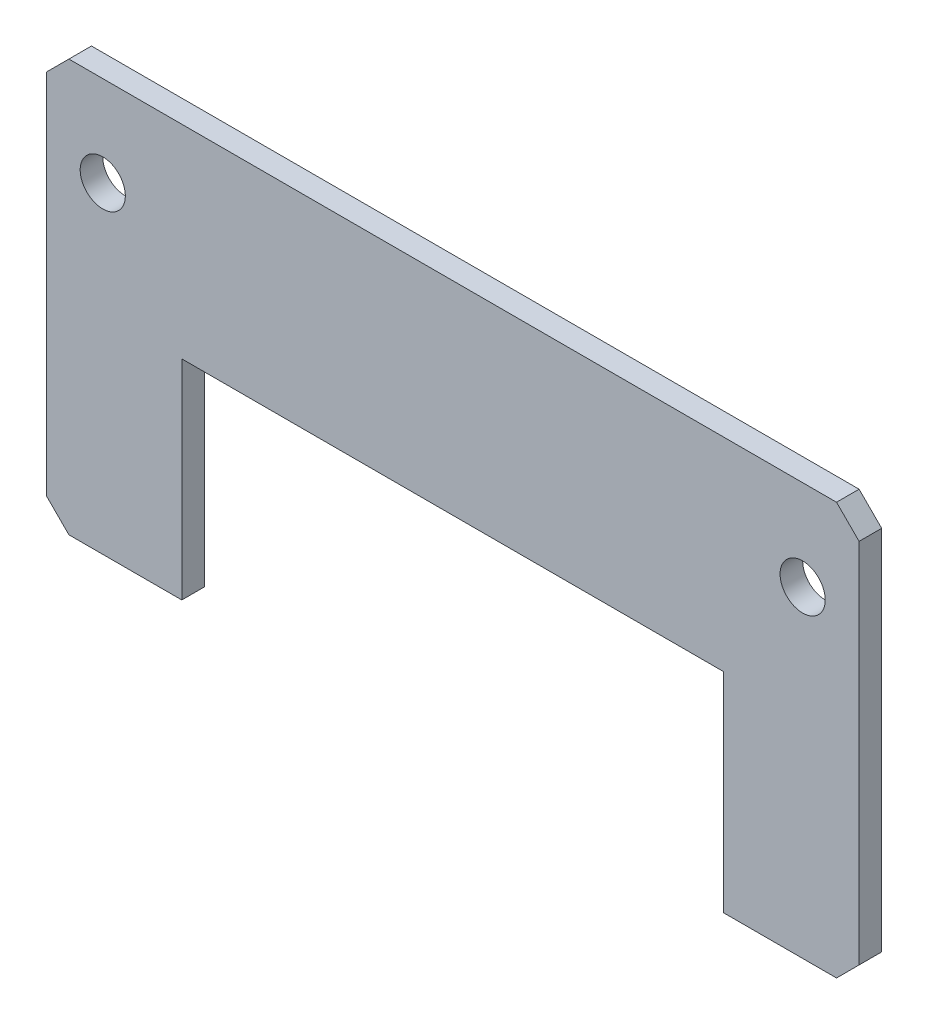
SolidWorks part; units mm, degrees
ref_plane "Front Plane" through (0, 0, 0) normal (0, 0, 1) x (1, 0, 0)
ref_plane "Top Plane" through (0, 0, 0) normal (0, 1, 0) x (1, 0, 0)
ref_plane "Right Plane" through (0, 0, 0) normal (1, 0, 0) x (0, 0, -1)
sketch "Sketch1" plane through (0, 0, 0) normal (0, 0, 1) x (1, 0, 0)
  line L1 (-360, 182.5) -> (360, 182.5)
  line L2 (-360, 182.5) -> (-360, -182.5)
  line L3 (-360, -182.5) -> (360, -182.5)
  line L4 (360, 182.5) -> (360, -182.5)
  line L5 (-360, 182.5) -> (360, -182.5) construction
  line L6 (-360, -182.5) -> (360, 182.5) construction
  point P0 (0, 0)
  dimension "D1" = 720
  dimension "D2" = 365
extrude "Boss-Extrude1" add sketch "Sketch1" along normal blind 20
sketch "Sketch2" plane through (0, 0, 20) normal (0, 0, 1) x (1, 0, 0)
  line L0 (-360, 182.5) -> (-360, -182.5) construction
  line L1 (360, 182.5) -> (-360, 182.5) construction
  line L2 (0, 283.7084) -> (0, -263.2572) construction
  circle A0 centre (-310, 102.5) radius 20
  circle A1 centre (310, 102.5) radius 20
  dimension "D3" = 40
  dimension "D1" = 50
  dimension "D2" = 80
extrude "Cut-Extrude1" cut sketch "Sketch2" against normal through all both and the other way through all
chamfer "Chamfer1" distance 20 angle 45 2 edges at (-360, 182.5, 10) (360, 182.5, 10)
chamfer "Chamfer2" distance 20 angle 45 2 edges at (360, -182.5, 10) (-360, -182.5, 10)
sketch "Sketch4" plane through (0, 0, 20) normal (0, 0, 1) x (1, 0, 0)
  line L0 (-340, -182.5) -> (340, -182.5) construction
  line L1 (-240, 2.5) -> (240, 2.5)
  line L2 (-240, 2.5) -> (-240, -367.5)
  line L3 (-240, -367.5) -> (240, -367.5)
  line L4 (240, 2.5) -> (240, -367.5)
  line L5 (-240, 2.5) -> (240, -367.5) construction
  line L6 (-240, -367.5) -> (240, 2.5) construction
  point P0 (0, -182.5)
  dimension "D1" = 480
  dimension "D2" = 185
extrude "Cut-Extrude2" cut sketch "Sketch4" against normal through all both and the other way through all
